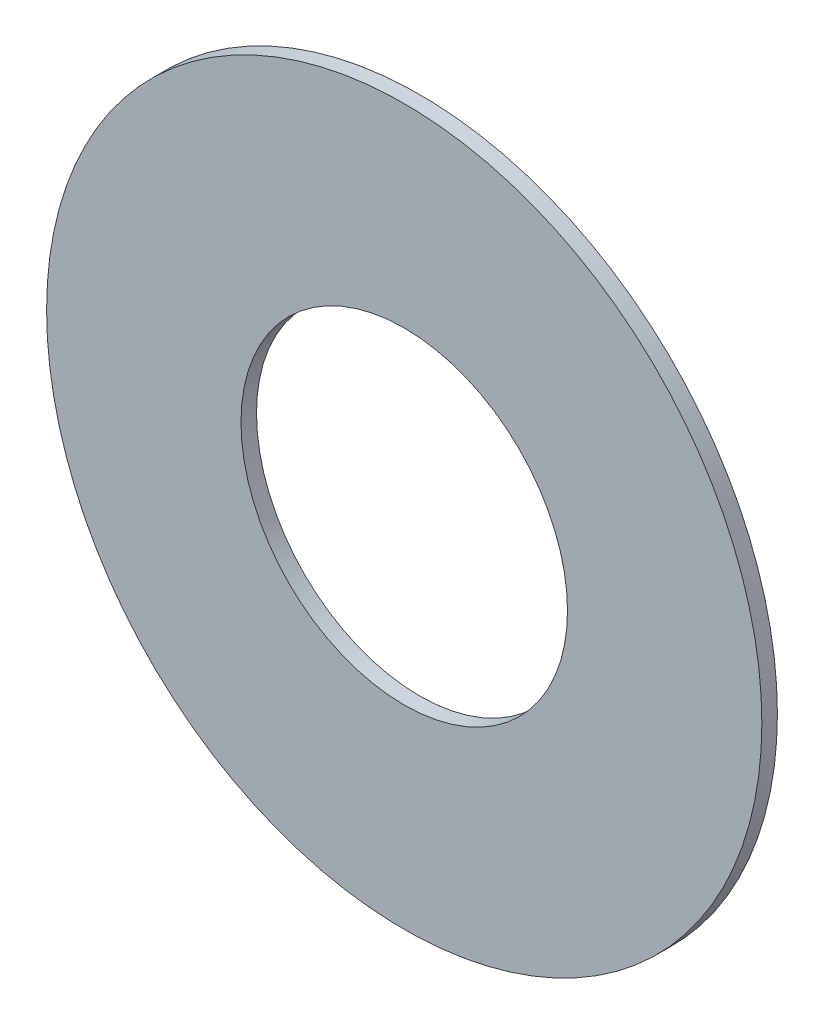
from build123d import *

# Parameters (mm, degrees)
SKETCH_1_R      = 23
SKETCH_1_R_2    = 10.5
EXTRUDE_1_DEPTH = 1


with BuildPart() as part:
    # 草图1 → 凸台-拉伸1 (new body)
    with BuildSketch(Plane.XY):
        Circle(SKETCH_1_R)
        Circle(SKETCH_1_R_2, mode=Mode.SUBTRACT)
    extrude(amount=EXTRUDE_1_DEPTH)


solid = part.part
